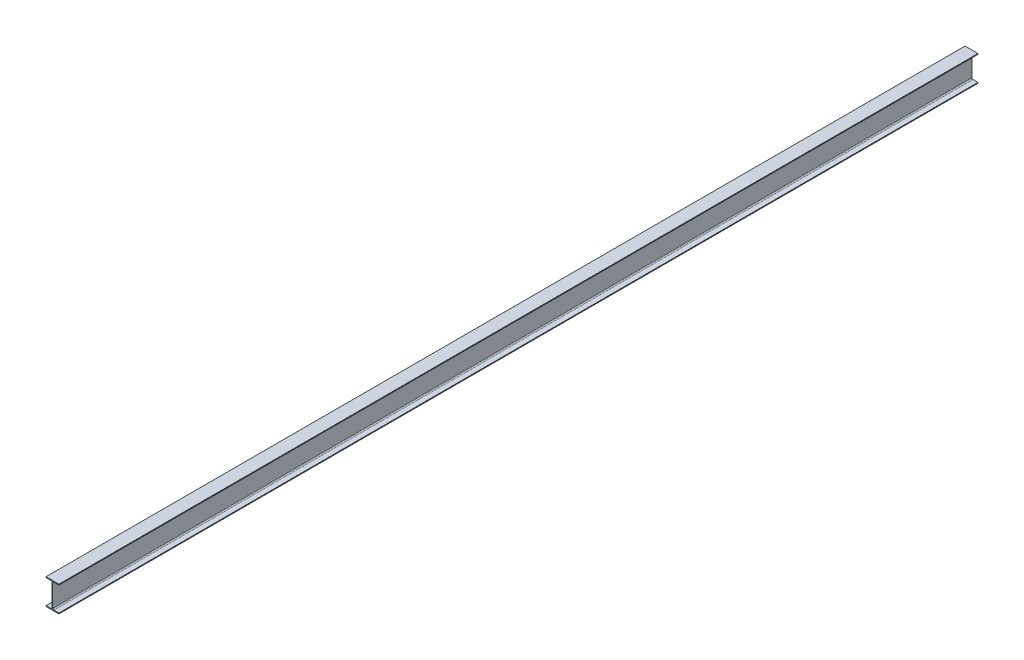
SolidWorks part; units mm, degrees
ref_plane "Front Plane" through (0, 0, 0) normal (0, 0, 1) x (1, 0, 0)
ref_plane "Top Plane" through (0, 0, 0) normal (0, 1, 0) x (1, 0, 0)
ref_plane "Right Plane" through (0, 0, 0) normal (1, 0, 0) x (0, 0, -1)
other "Configuration Table"
sketch "Sketch1" plane through (0, 0, 0) normal (0, 0, 1) x (1, 0, 0)
  line L0 (0, 0) -> (0, 300) construction
  line L1 (75, 0) -> (-75, 0)
  line L2 (-75, 0) -> (-75, 9)
  line L3 (-75, 9) -> (-16.25, 9)
  line L4 (3.25, 22) -> (3.25, 278)
  line L6 (-75, 291) -> (-75, 300)
  line L7 (-75, 300) -> (75, 300)
  line L8 (-3.25, 22) -> (-3.25, 278)
  line L9 (75, 291) -> (75, 300)
  line L10 (16.25, 291) -> (75, 291)
  line L11 (75, 9) -> (16.25, 9)
  line L12 (75, 0) -> (75, 9)
  line L13 (-16.25, 291) -> (-75, 291)
  arc A0 (16.25, 9) -> (3.25, 22) centre (16.25, 22) cw
  arc A1 (-3.25, 22) -> (-16.25, 9) centre (-16.25, 22) cw
  arc A2 (3.25, 278) -> (16.25, 291) centre (16.25, 278) cw
  arc A3 (-3.25, 278) -> (-16.25, 291) centre (-16.25, 278) ccw
  point P18 (3.25, 9)
  point P21 (-3.25, 9)
  point P24 (3.25, 291)
  point P27 (-3.25, 291)
  dimension "D6" = 13
  dimension "D1" = 300
  dimension "D2" = 150
  dimension "D3" = 6.5
  dimension "D4" = 9
  dimension "D5" = 9
extrude "Boss-Extrude1" add sketch "Sketch1" along normal blind 10687
